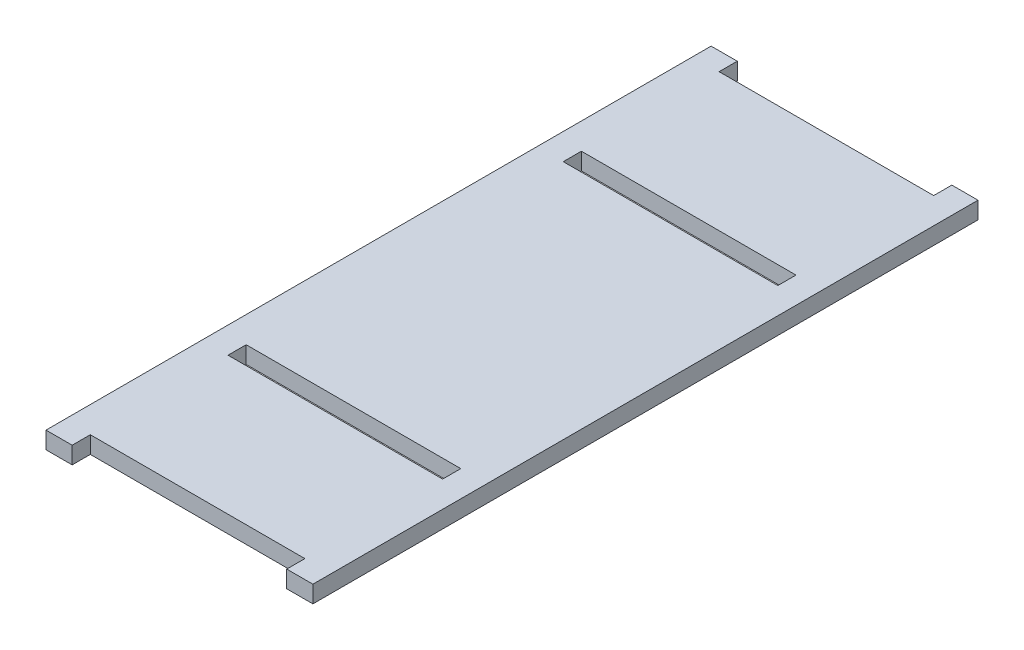
SolidWorks part; units mm, degrees
material "Q235B"
ref_plane "Front Plane" through (0, 0, 0) normal (0, 0, 1) x (1, 0, 0)
ref_plane "Top Plane" through (0, 0, 0) normal (0, 1, 0) x (1, 0, 0)
ref_plane "Right Plane" through (0, 0, 0) normal (1, 0, 0) x (0, 0, -1)
other "Configuration Table"
sketch "Sketch1" plane through (0, 0, 0) normal (0, 1, 0) x (1, 0, 0)
  line L0 (0, 0) -> (325.3094, 0) construction
  line L1 (-125, -311.5) -> (125, -311.5)
  line L2 (-125, -311.5) -> (-125, 311.5)
  line L3 (-125, 311.5) -> (125, 311.5)
  line L4 (125, -311.5) -> (125, 311.5)
  line L5 (-125, -311.5) -> (125, 311.5) construction
  line L6 (-125, 311.5) -> (125, -311.5) construction
  line L7 (-100.5, 311.5) -> (100.5, 311.5)
  line L8 (-100.5, 311.5) -> (-100.5, 294.5)
  line L9 (-100.5, 294.5) -> (100.5, 294.5)
  line L10 (100.5, 311.5) -> (100.5, 294.5)
  line L11 (-100.5, -311.5) -> (100.5, -311.5)
  line L12 (-100.5, -311.5) -> (-100.5, -294.5)
  line L13 (-100.5, -294.5) -> (100.5, -294.5)
  line L14 (100.5, -311.5) -> (100.5, -294.5)
  line L15 (-100.5, 165.5) -> (100.5, 165.5)
  line L16 (-100.5, 165.5) -> (-100.5, 148.5)
  line L17 (-100.5, 148.5) -> (100.5, 148.5)
  line L18 (100.5, 165.5) -> (100.5, 148.5)
  line L19 (-100.5, -148.5) -> (100.5, -148.5)
  line L20 (100.5, -165.5) -> (100.5, -148.5)
  line L21 (-100.5, -165.5) -> (100.5, -165.5)
  line L22 (-100.5, -165.5) -> (-100.5, -148.5)
  point P0 (0, 0)
  point P18 (0, 148.5)
  point P19 (0, 294.5)
  point P21 (0, -294.5)
  dimension "D1" = 250
  dimension "D2" = 623
  dimension "D3" = 589
  dimension "D4" = 165.5
  dimension "D5" = 17
  dimension "D6" = 201
  dimension "D7" = 201
  dimension "D8" = 201
  dimension "D9" = 0
  dimension "D10" = 0
  dimension "D11" = 0
extrude "Boss-Extrude1" add sketch "Sketch1" along normal blind 16 contours L14 L1 L4 L3 L10 L9 L8 L2 L12 L13 L15 L18 L17 L16 L21 L22 L19 L20
